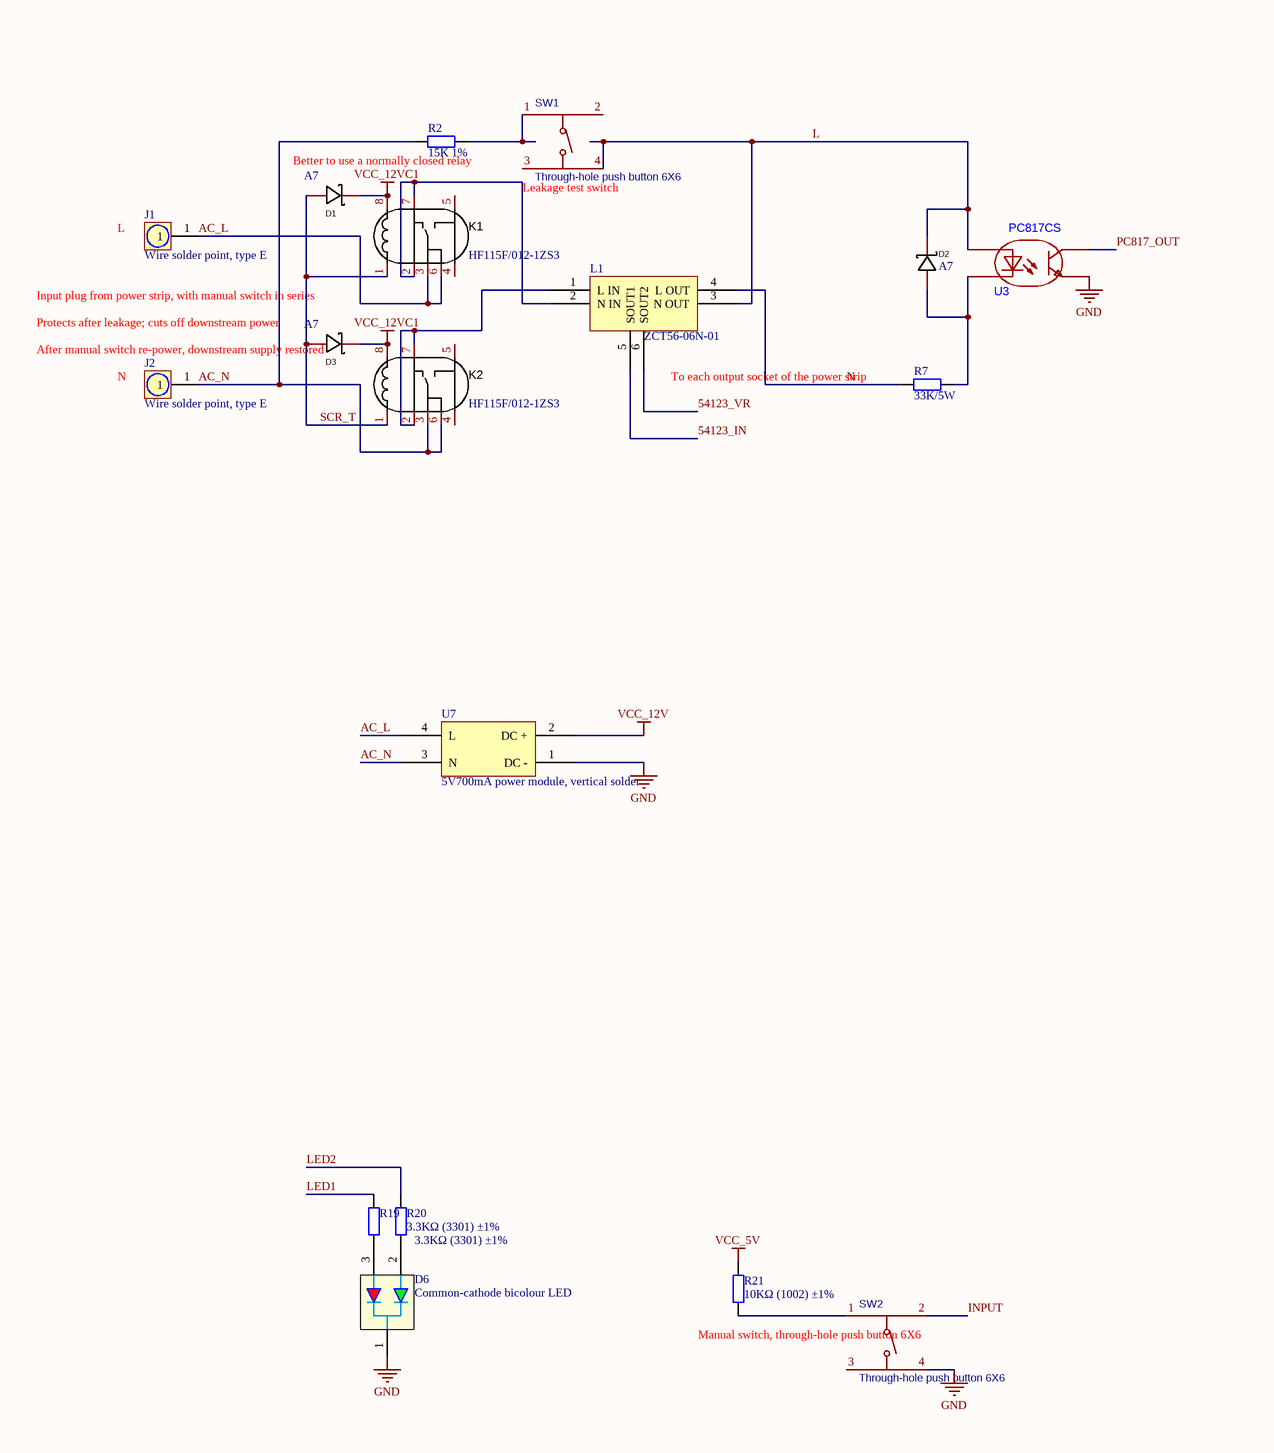
[diagram p0: MISC89365.SchDoc, left]
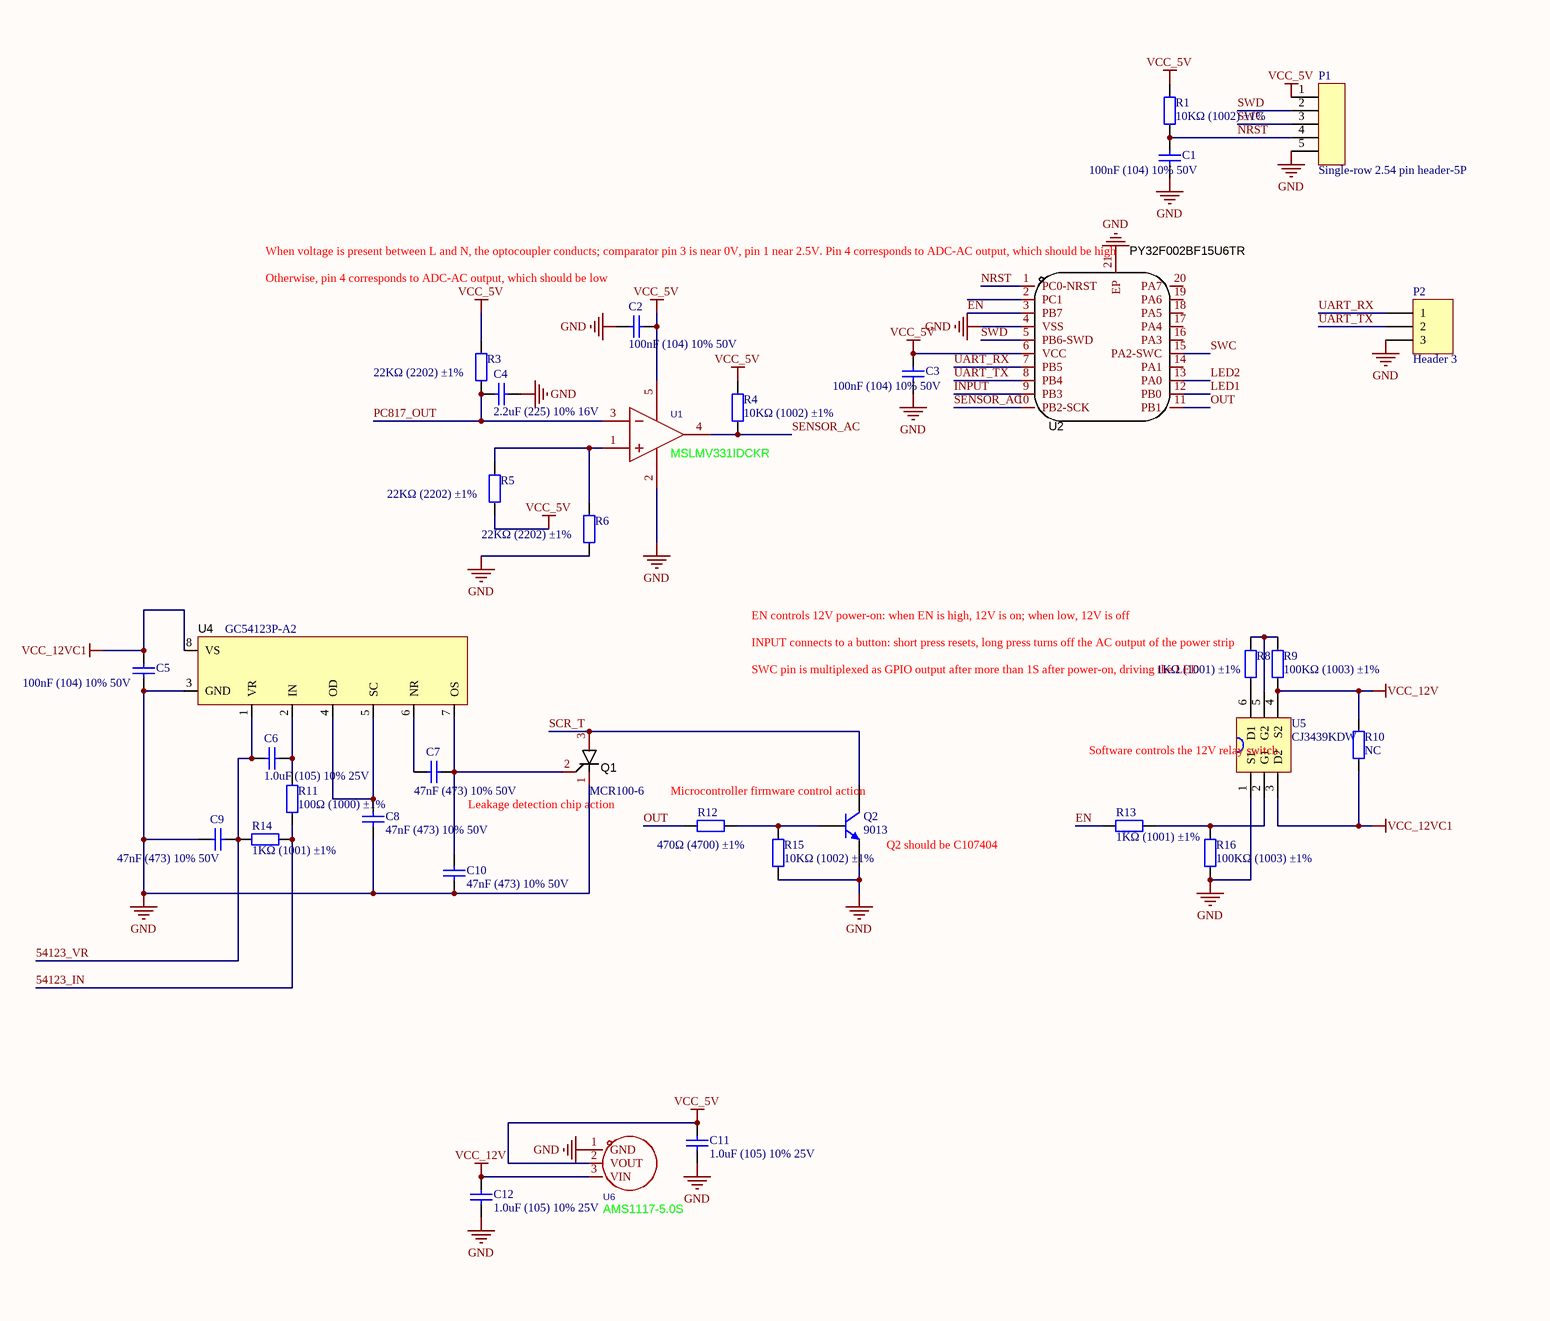
[diagram p1: MISC89365.SchDoc, right]
# Altium project MISC89365-7.PrjPCB
1 sheet, 53 parts. Net scope: global (net labels, ports and power ports of the same name join across sheets).
Board file: MISC89365.PcbDoc

## Sheet MISC89365.SchDoc
size A2

### Parts
C1  100nF (104) 10% 50V  [0402_C]
C2  100nF (104) 10% 50V  [0402_C]
C3  100nF (104) 10% 50V  [0402_C]
C4  2.2uF (225) 10% 16V  [0603_C]
C5  100nF (104) 10% 50V  [0402_C]
C6  1.0uF (105) 10% 25V  [0402_C]
C7  47nF (473) 10% 50V  [0402_C]
C8  47nF (473) 10% 50V  [0402_C]
C9  47nF (473) 10% 50V  [0402_C]
C10  47nF (473) 10% 50V  [0402_C]
C11  1.0uF (105) 10% 25V  [0402_C]
C12  1.0uF (105) 10% 25V  [0402_C]
D1  A7  [SOD-123FL_L2.8-W1.8-LS3.7-RD]
D2  A7  [SOD-123FL_L2.8-W1.8-LS3.7-RD]
D3  A7  [SOD-123FL_L2.8-W1.8-LS3.7-RD]
D6  Common-cathode bicolour LED  [LED 3MM-2P]
J1  Wire solder point, type E  [焊线点E型]
J2  Wire solder point, type E  [焊线点E型]
K1  HF115F/012-1ZS3  [RELAY-TH_HF115F-012-1ZS3]
K2  HF115F/012-1ZS3  [RELAY-TH_HF115F-012-1ZS3]
L1  ZCT56-06N-01  [ZCT56-06N-01]
P1  Single-row 2.54 pin header-5P  [HDR1X5]
P2  Header 3  [HDR1X3]
Q1  MCR100-6  [SOT-23-3_L2.9-W1.3-P1.90-LS2.4-BR]
Q2  9013  [SOT-23(SOT-23-3)]
R1  10KΩ (1002) ±1%  [0402_R]
R2  15K 1%  [1210_R]
R3  22KΩ (2202) ±1%  [0402_R]
R4  10KΩ (1002) ±1%  [0402_R]
R5  22KΩ (2202) ±1%  [0402_R]
R6  22KΩ (2202) ±1%  [0402_R]
R7  33K/5W  [5W直插电阻横插]
R8  1KΩ (1001) ±1%  [0402_R]
R9  100KΩ (1003) ±1%  [0402_R]
R10  NC  [0603_R]
R11  100Ω (1000) ±1%  [0402_R]
R12  470Ω (4700) ±1%  [0402_R]
R13  1KΩ (1001) ±1%  [0402_R]
R14  1KΩ (1001) ±1%  [0402_R]
R15  10KΩ (1002) ±1%  [0402_R]
R16  100KΩ (1003) ±1%  [0402_R]
R19  3.3KΩ (3301) ±1%  [0402_R]
R20  3.3KΩ (3301) ±1%  [0402_R]
R21  10KΩ (1002) ±1%  [0402_R]
SW1  Through-hole push button 6X6  [SW-TH_4P-L6.0-W6.0-P4.50-LS6.5]
SW2  Through-hole push button 6X6  [SW-TH_4P-L6.0-W6.0-P4.50-LS6.5]
U1  MSLMV331IDCKR  [SC-70-5_L2.1-W1.3-P0.65-LS2.3-BL]
U2  PY32F002BF15U6TR  [QFN-20_L3.0-W3.0-P0.40-TL-EP1.7]
U3  PC817CS  [SOP-4_L6.5-W4.6-P2.54-LS10.2-BL]
U4  GC54123P-A2  [SOP-8_L5.0-W4.0-P1.27-LS6.2-BL]
U5  CJ3439KDW  [SOT-363]
U6  AMS1117-5.0S  [SOT-89-3_L4.5-W2.5-P1.50-LS4.2-BR]
U7  5V700mA power module, vertical solder  [5V700mA电源模块竖直焊接]

### Nets
GND: C1.2 C2.2 C3.2 C4.2 C5.1 C8.1 C9.1 C10.1 C11.1 C12.1 D6.1 P1.5 P2.3 Q1.1(K) Q2.2(E) R6.1 R15.1 R16.1 SW2.4 U1.2(V-) U2.4(VSS) U2.21(EP) U3.3(Emitter) U4.3(GND) U5.1(S1) U6.1(GND) U7.1(DC_-)
VCC_5V: C2.1 C3.1 C11.2 P1.1 R1.2 R3.2 R4.2 R5.1 R21.2 U1.5(V+) U2.6(VCC) U6.2(VOUT)
VCC_12V: C12.2 R9.1 R10.2 U5.4(S2) U6.3(VIN) U7.2(DC_+)
VCC_12VC1: C5.2 D1.1(K) D3.1(K) K1.8 K2.8 R10.1 U4.8(VS) U5.3(D2)
54123_IN: L1.5(SOUT1) R11.1 R14.2
54123_VR: C6.2 C9.2 L1.6(SOUT2) R14.1 U4.1(VR)
AC_L: J1.1 K1.3 K1.6 U7.4(L)
AC_N: J2.1 K2.3 K2.6 R2.1 U7.3(N)
EN: R13.1 U2.3(PB7)
INPUT: SW2.2 U2.9(PB3)
L: D2.1(K) L1.3(N_OUT) SW1.4 U3.1(Anode)
LED1: R19.2 U2.12(PB0)
LED2: R20.2 U2.13(PA0)
N: L1.4(L_OUT) R7.1
NRST: C1.1 P1.4 R1.1 U2.1(PC0-NRST)
OUT: R12.1 U2.11(PB1)
PC817_OUT: C4.1 R3.1 U1.3(IN-) U3.4(Collector)
SCR_T: D1.2(A) D3.2(A) K1.1 K2.1 Q1.3(A) Q2.3(C)
SENSOR_AC: R4.1 U1.4(OUT) U2.10(PB2-SCK)
SWC: P1.3 U2.15(PA2-SWC)
SWD: P1.2 U2.5(PB6-SWD)
UART_RX: P2.1 U2.7(PB5)
UART_TX: P2.2 U2.8(PB4)
NetC6_1: C6.1 R11.2 U4.2(IN)
NetC7_1: C7.1 U4.6(NR)
NetC7_2: C7.2 C10.2 Q1.2(G) U4.7(OS)
NetC8_2: C8.2 U4.4(OD) U4.5(SC)
NetD2_2: D2.2(A) R7.2 U3.2(Cathode)
NetD6_2: D6.2 R20.1
NetD6_3: D6.3 R19.1
NetK1_2: K1.2 K1.7 L1.2(N_IN)
NetK2_2: K2.2 K2.7 L1.1(L_IN)
NetQ2_1: Q2.1(B) R12.2 R15.2
NetR2_2: R2.2 SW1.1
NetR5_2: R5.2 R6.2 U1.1(IN+)
NetR8_1: R8.1 U5.6(D1)
NetR8_2: R8.2 R9.2 U5.5(G2)
NetR13_2: R13.2 R16.2 U5.2(G1)
NetR21_1: R21.1 SW2.1

Not connected (* = marked no-connect by the designer): K1 4 5; K2 4 5; SW1 2 3; SW2 3; U2 2(PC1) 14(PA1) 16(PA3) 17(PA4) 18(PA5) 19(PA6) 20(PA7)

### Notes on the sheet
- (near U2) When voltage is present between L and N, the optocoupler conducts; comparator pin 3 is near 0V, pin 1 near 2.5V. Pin 4 corresponds to ADC-AC output, which should be high
- (near C2) Otherwise, pin 4 corresponds to ADC-AC output, which should be low
- Better to use a normally closed relay
- (near SW1) Leakage test switch
- (near J1) L
- Input plug from power strip, with manual switch in series
- (near D3) Protects after leakage; cuts off downstream power
- (near D3) After manual switch re-power, downstream supply restored
- (near J2) N
- (near R7) To each output socket of the power strip
- EN controls 12V power-on: when EN is high, 12V is on; when low, 12V is off
- INPUT connects to a button: short press resets, long press turns off the AC output of the power strip
- SWC pin is multiplexed as GPIO output after more than 1S after power-on, driving the LED
- (near U5) Software controls the 12V relay switch
- Leakage detection chip action
- (near Q2) Microcontroller firmware control action
- (near Q2) Q2 should be C107404
- (near SW2) Manual switch, through-hole push button 6X6

### Library data of the parts
C1-C3 C5 = 0402 100nF (104) 10% 50V: SMD capacitor; ComponentLink1Description: Supplier link; Package: 0402; Supplier: LC; SuppliersPartNumber: C77020
C4 = 0603 2.2uF (225) 10% 16V: SMD capacitor; ComponentLink1Description: Supplier link; Package: 0603; Supplier: LC; SuppliersPartNumber: C23630
C6 C11 C12 = 0402 1.0uF (105) 10% 25V: SMD capacitor; ComponentLink1Description: Supplier link; Package: 0402; Supplier: LC; SuppliersPartNumber: C52923
C7-C10 = 0402 47nF (473) 10% 50V: SMD capacitor; ComponentLink1Description: Supplier link; Package: 0402; Supplier: LC; SuppliersPartNumber: C272875
D1-D3 = A7: General-purpose diode; Manufacturer: GOODWORK(固得沃克); Symbol: A7_C2891324; Add into BOM: yes; Diode Configuration: Standalone; Reverse Voltage (Vr): 1kV; Average Rectified Current (Io): 1A; Forward Voltage (Vf@If): 1.1V@1A; Reverse Leakage Current: 5μA@1kV; Name: A7; Device: A7_C2891324; LCSC Part Name: 1kV 1A 1.1V@1A; SuppliersPartNumber: C2891324; Manufacturer Part: A7; Supplier Footprint: SOD123FL; JLCPCB Part Class: Extended Part; Datasheet: https://example.com/upload/public/pdf/source/20210903/C6D4BE94189732442E7E9701A5BFE16D.pdf; Supplier: LC; Convert to PCB: yes
D6 = LED 3MM-2P共阴: Bicolour LED red+green; SuppliersPartNumber: C72703; Supplier: LC
J1 J2 = 焊线点E型: Wire solder joint, hole diameter about 3mm; Suppliers: ATE; SuppliersPartNumber: ATE
K1 K2 = HF115F/012-1ZS3: Single changeover (SPDT); Manufacturer: HF(宏发); Add into BOM: yes; Coil Voltage: 12V; Coil Type: Non-polarised, single coil; Pin Number: 8; Contact Form: Single changeover:1C (SPDT); Maximum Switching Current: 16A; Maximum Switching Voltage: 440V@AC; 300V@DC; Coil Rated Power: 400mW; Contact Rating: 16A@250VAC; Coil Resistance: 360Ω; Operate Time: 15ms; Release Time: 8ms; Contact Resistance: 100mΩ; Name: HF115F/012-1ZS3; Symbol: HF115F/012-1ZS3; Device: HF115F/012-1ZS3; LCSC Part Name: 小型大功率直流12V继电器 单刀双掷; SuppliersPartNumber: C329299; Manufacturer Part: HF115F/012-1ZS3; Supplier Footprint: DIP,12.7x29mm; JLCPCB Part Class: Extended Part; Datasheet: https://example.com/upload/public/pdf/source/20181114/C329299_11AFA41C509BE74E6FC0D9576B429905.pdf; Supplier: LC; Convert to PCB: yes; Contact Material: AgCdO; Operating Temperature: -40℃~+85℃
L1 = ZCT56-06N-01: Miniature solder-pad zero-sequence sensor; Supplier: *; SuppliersPartNumber: *
P1 = 单排2.54排针-5P
P2 = Header 3: Header, 3-Pin; LatestRevisionDate: 17-Jul-2002; LatestRevisionNote: Re-released for DXP Platform.; Publisher: Altium Limited
Q1 = MCR100-6: 0.8A unidirectional thyristor; Manufacturer: CBI(创基); Symbol: MCR100-6 100-6; Device: MCR100-6_C2919773; Add into BOM: yes; Name: MCR100-6; LCSC Part Name: MCR100-6 100-6; SuppliersPartNumber: C5155446; Manufacturer Part: MCR100-6; Supplier Footprint: SOT-23; JLCPCB Part Class: Extended Part; Datasheet: https://example.com/upload/public/pdf/source/20211122/0F9C7AE0191D7A6CB122BB5125AF119E.pdf; Supplier: LC; Convert to PCB: yes
Q2 = SOT-23 9013: Transistor; ComponentLink1Description: Supplier link; Package: SOT-23; Supplier: LC; SuppliersPartNumber: C81408
R1 R4 R15 R21 = 0402 10KΩ (1002) 1%: SMD resistor; ComponentLink1Description: Supplier link; Package: 0402; Supplier: LC; SuppliersPartNumber: C25744
R2 = 1210 15K 1%: SMD resistor; ComponentLink1Description: Supplier link; Package: 1210; Supplier: LC; SuppliersPartNumber: C874731
R3 R5 R6 = 0402 22KΩ (2202) 1%: SMD resistor; ComponentLink1Description: Supplier link; Package: 0402; Supplier: LC; SuppliersPartNumber: C25768
R7 = 33K/5W: 5W through-hole resistor; ComponentLink1Description: Supplier link; Package: 5W; Supplier: TB; SuppliersPartNumber: *
R8 R13 R14 = 0402 1KΩ (1001) 1%: SMD resistor; ComponentLink1Description: Supplier link; Package: 0402; Supplier: LC; SuppliersPartNumber: C11702
R9 R16 = 0402 100KΩ (1003) 1%: SMD resistor; ComponentLink1Description: Supplier link; Package: 0402; Supplier: LC; SuppliersPartNumber: C25741
R10 = 0603 0Ω (0R0) 1%: SMD resistor; ComponentLink1Description: Supplier link; Package: 0603; Supplier: LC; SuppliersPartNumber: C21189
R11 = 0402 100Ω (1000) 1%: SMD resistor; ComponentLink1Description: Supplier link; Package: 0402; Supplier: LC; SuppliersPartNumber: C25076
R12 = 0402 470Ω (4700) 1%: SMD resistor; ComponentLink1Description: Supplier link; Package: 0402; Supplier: LC; SuppliersPartNumber: C25117
R19 R20 = 0402 3.3KΩ (3301) 1%: SMD resistor; ComponentLink1Description: Supplier link; Package: 0402; Supplier: LC; SuppliersPartNumber: C25890
SW1 SW2 = 直插按键6X6: BOM_Manufacturer: Yuandi; BOM_Manufacturer Part: TS-1095-A3B2-D1; Contributor: LCSC; Supplier: LC; SuppliersPartNumber: C782806; BOM_JLCPCB Part Class: Extended Part; spicePre: S; spiceSymbolName: TS-1095-A3B2-D1
U1 = MSLMV331IDCKR: Single-channel comparator; Symbol: MSLMV331IDCKR; Supplier: LC; SuppliersPartNumber: C49208515
U2 = PY32F002BF15U6TR: PUYA M0 microcontroller; Manufacturer: PUYA(普冉); Add into BOM: yes; Symbol: PY32F002BF15U6TR; Device: PY32F002BF15U6TR; LCSC Part Name: PY32F002BF15U6TR; SuppliersPartNumber: C7469099; Manufacturer Part: PY32F002BF15U6TR; Supplier Footprint: QFN-20-EP(3x3); JLCPCB Part Class: Extended Part; Datasheet: https://example.com/upload/public/pdf/source/20230721/558A839BF110561168DB9B6F0054F7DC.pdf; Supplier: LC; Convert to PCB: yes; Comment_1: PY32F002BF15U6TR
U3 = PC817CS: Optocoupler; Manufacturer: AOTE(奥特); Add into BOM: yes; Input voltage type: DC; Output Type: Phototransistor; Forward Voltage: 1.2V; Output Current: 50mA; Isolation Voltage(rms): 5kV; Reverse Voltage: 6V; Number of Outputs: 1; Collector-Emitter Saturation Voltage (Vce(sat)@Ic,IF): 200mV@1mA,20mA; Rise time: 4us; Fall time: 3us; Symbol: PC817CS; Device: PC817CS; LCSC Part Name: 光耦-光电晶体管输出; SupplierPartNumber: C20612591; Manufacturer Part: PC817CS; Supplier Footprint: SOP-4; JLCPCB Part Class: Extended Part; Datasheet: https://example.com/upload/public/pdf/source/20240430/65190B5F12AF4832AD866CBB877395F1.pdf; Supplier: LC; Convert to PCB: yes; Operating Temperature: -55℃~+110℃
U4 = GC54123P-A2: Leakage protection; Manufacturer: 鑫雁; Add into BOM: yes; Name: GC54123P-A2; Symbol: GC54123P-A2; Device: GC54123P-A2; LCSC Part Name: GC54123P-A2; SuppliersPartNumber: C2683253; Manufacturer Part: GC54123P-A2; Supplier Footprint: SOP-8; JLCPCB Part Class: Extended Part; Datasheet: https://example.com/upload/public/pdf/source/20210120/C2683253_E7524B42559DF5FD9458CD53AECDAB62.pdf; Supplier: LC; Convert to PCB: yes
U5 = CJ3439KDW: NMOS+PMOS; Supplier: LC; SuppliersPartNumber: C99824
U6 = AMS1117-5.0S: Symbol: AMS1117-5.0S_C46473006; Supplier: LC; SuppliersPartNumber: C46473006
U7 = 5V700mA电源模块竖直焊接: Supplier: *; SupplierPartNumber: *